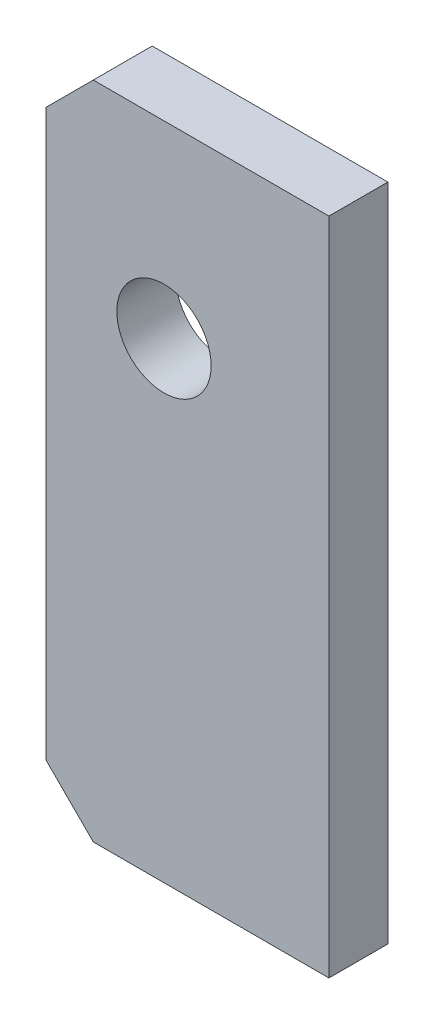
from build123d import *

# Parameters (mm, degrees)
SKETCH_1_W               = 120
SKETCH_1_H               = 280
EXTRUDE_1_DEPTH          = 25
CUT_EXTRUDE_1_DEPTH      = 306.655034312
CUT_EXTRUDE_1_DEPTH_BACK = 306.655034312
SKETCH_2_R               = 20
CHAMFER_1_SIZE           = 20


with BuildPart() as part:
    # 草图1 → 凸台-拉伸1 (new body)
    with BuildSketch(Plane.XY):
        with Locations((-60, 140)):
            Rectangle(SKETCH_1_W, SKETCH_1_H)
    extrude(amount=EXTRUDE_1_DEPTH)

    # 草图2 → 切除-拉伸1 (cut, two sides: drawn at the far end of the back side and taken through both)
    with BuildSketch(Plane.XY.offset(25).offset(-CUT_EXTRUDE_1_DEPTH_BACK)):
        with Locations((-70, 200)):
            Circle(SKETCH_2_R)
    extrude(amount=CUT_EXTRUDE_1_DEPTH + CUT_EXTRUDE_1_DEPTH_BACK, mode=Mode.SUBTRACT)

    # 倒角1
    chamfer_1_edges = [part.edges().sort_by_distance(p)[0] for p in [
        (-120, 0, 12.5),
        (-120, 280, 12.5),
    ]]
    chamfer(chamfer_1_edges, length=CHAMFER_1_SIZE)


solid = part.part
